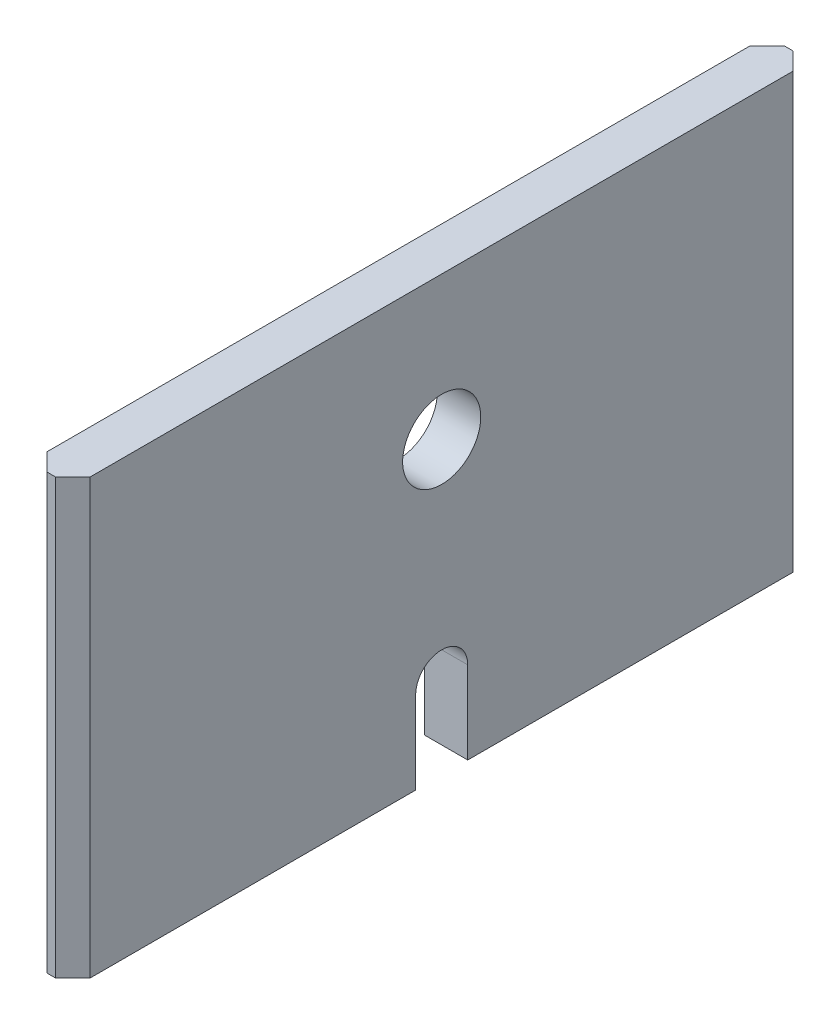
from build123d import *

# Parameters (mm, degrees)
SKETCH1_R           = 45
BOSS_EXTRUDE1_DEPTH = 25
CHAMFER1_SIZE       = 20


with BuildPart() as part:
    # Sketch1 → Boss-Extrude1 (new, symmetric)
    with BuildSketch(Plane(origin=(0, 0, 0), x_dir=(0, 0, -1), z_dir=(1, 0, 0))):
        with BuildLine():
            Line((425, -250), (30, -250))
            Line((30, -250), (30, -155))
            ThreePointArc((30, -155), (0, -125), (-30, -155))
            Line((-30, -155), (-30, -250))
            Line((-30, -250), (-425, -250))
            Line((-425, -250), (-425, 250))
            Line((-425, 250), (425, 250))
            Line((425, 250), (425, -250))
        make_face()
        with Locations((0, 85)):
            Circle(SKETCH1_R, mode=Mode.SUBTRACT)
    extrude(amount=BOSS_EXTRUDE1_DEPTH, both=True)

    # Chamfer1
    chamfer1_edges = [part.edges().sort_by_distance(p)[0] for p in [
        (-25, 0, 425),
        (25, 0, -425),
        (25, 0, 425),
        (-25, 0, -425),
    ]]
    chamfer(chamfer1_edges, length=CHAMFER1_SIZE)


solid = part.part
